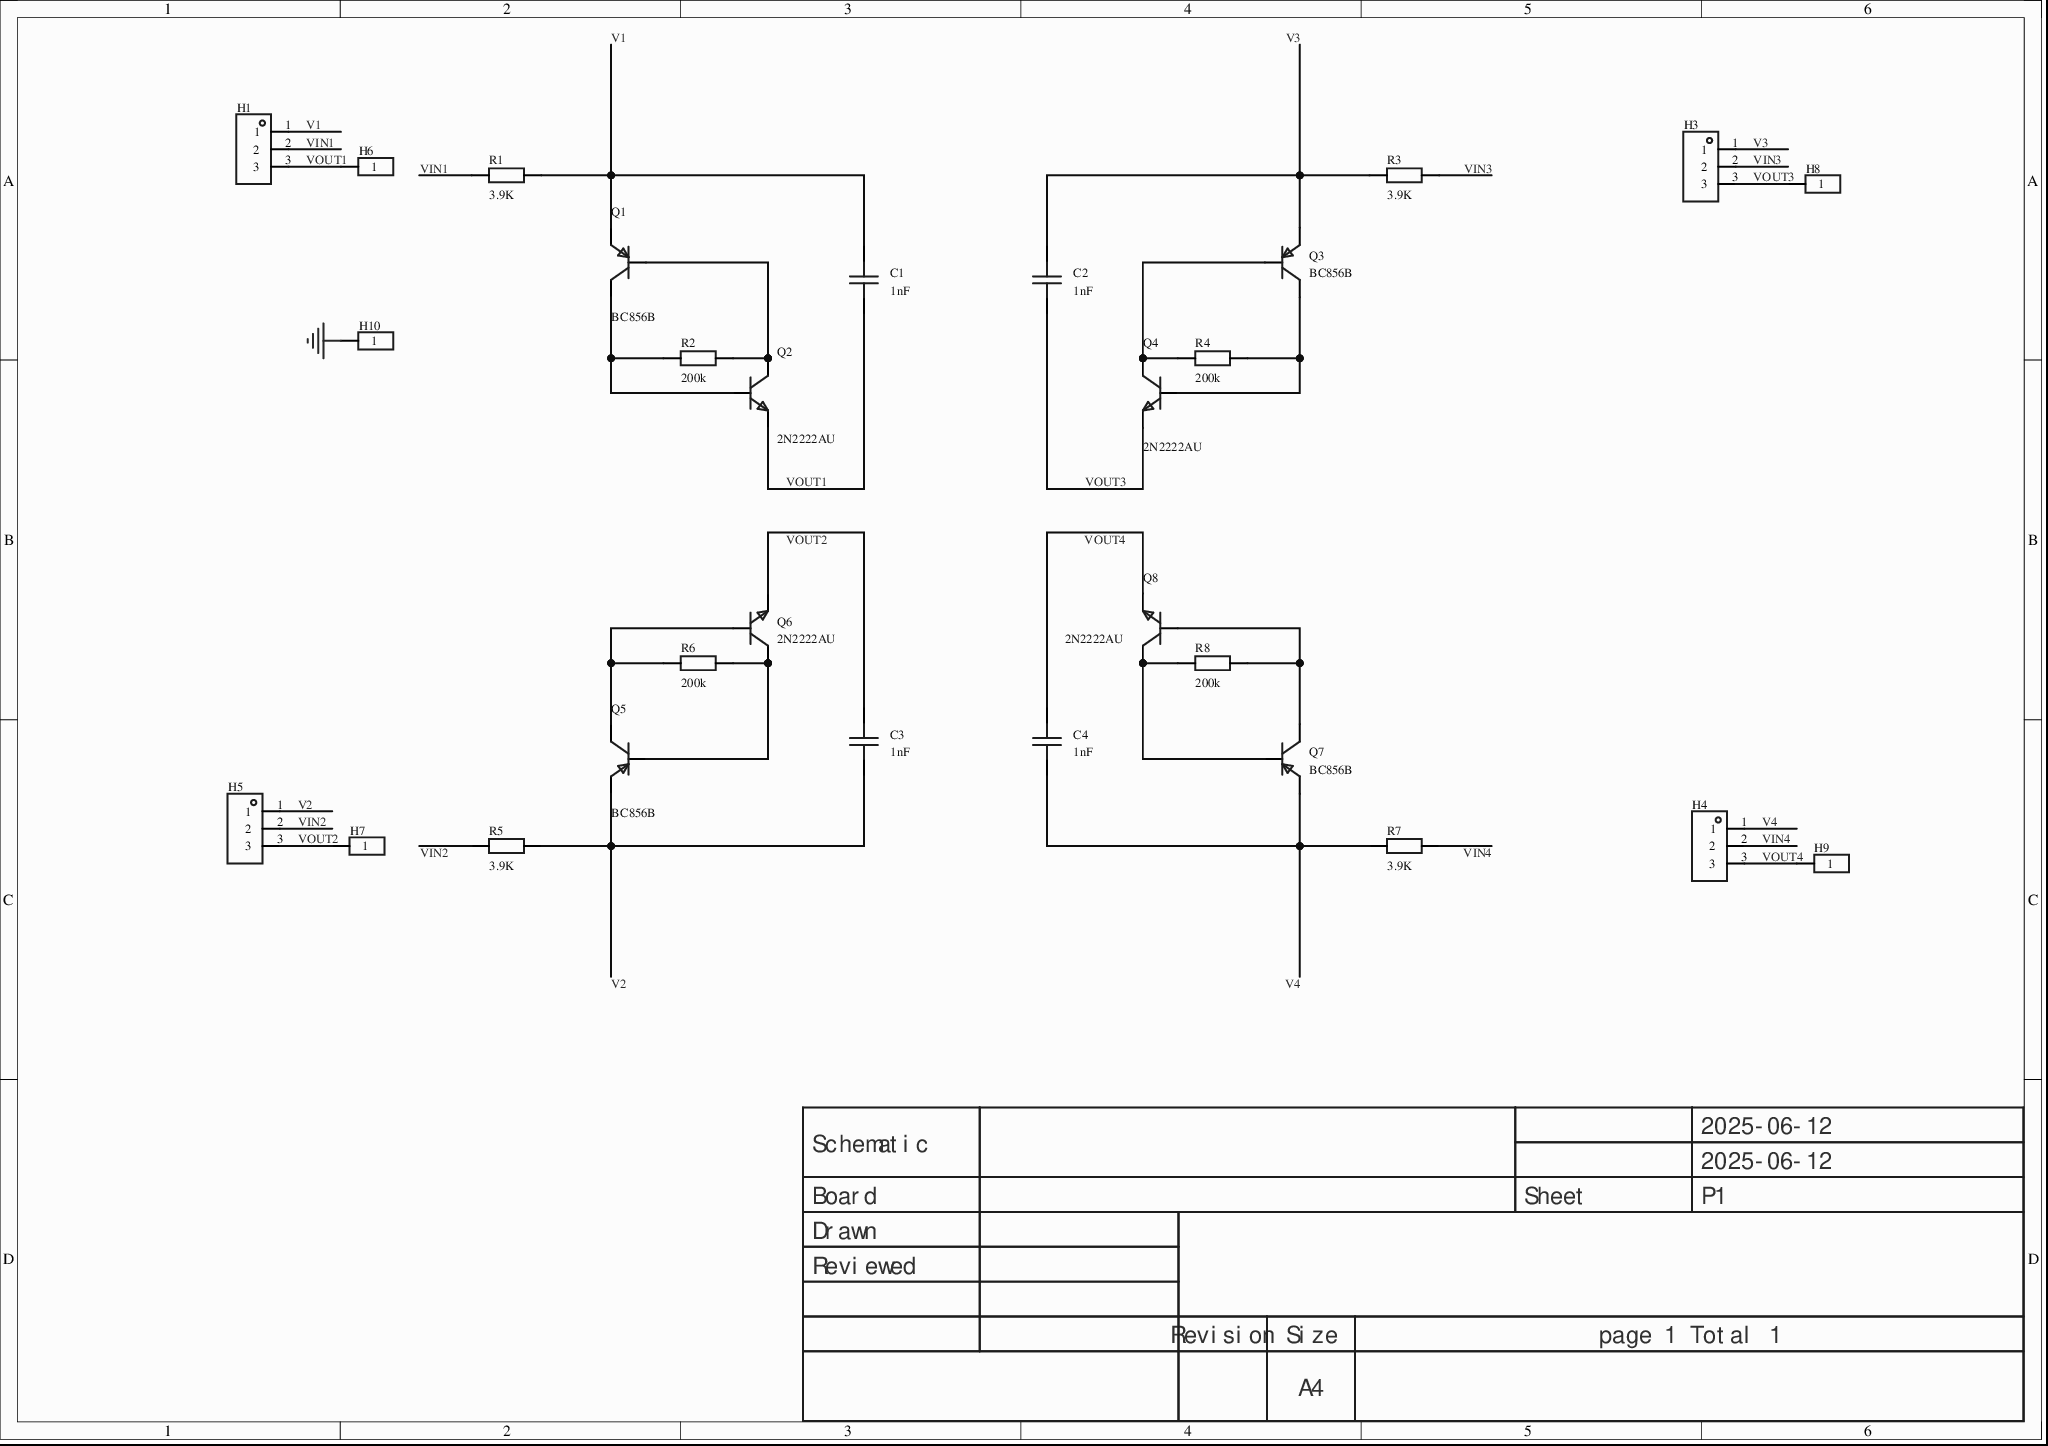
[diagram p0: MISC51650-3.schdoc]
# Altium project MISC51650-2.PrjPcb
1 sheet, 29 parts. Net scope: global (net labels, ports and power ports of the same name join across sheets).
Board file: MISC51650.pcbdoc

## Sheet MISC51650-3.schdoc
size 297 x 209 mm; Version: V1.0; @Project Name: MISC51650; @Page Count: 1; @Update Date: 2025-06-12; @Create Date: 2025-06-12; @Schematic Name: MISC51650; @Page No: 1; @Create Time: 12:37:26; @Update Time: 12:37:29; @Board Name: MISC51650

### Parts
C1  1nF  [C0402]
C2  1nF  [C0402]
C3  1nF  [C0402]
C4  1nF  [C0402]
H1  (no value)  [HDR-TH_2P-P2.54-V-M-1]
H3  (no value)  [HDR-TH_2P-P2.54-V-M-1]
H4  (no value)  [HDR-TH_2P-P2.54-V-M-1]
H5  (no value)  [HDR-TH_2P-P2.54-V-M-1]
H6  (no value)  [HDR-TH_1P-V-M_XKB_X4611WV-01I-C28D40]
H7  (no value)  [HDR-TH_1P-V-M_XKB_X4611WV-01I-C28D40]
H8  (no value)  [HDR-TH_1P-V-M_XKB_X4611WV-01I-C28D40]
H9  (no value)  [HDR-TH_1P-V-M_XKB_X4611WV-01I-C28D40]
H10  (no value)  [HDR-TH_1P-V-M_XKB_X4611WV-01I-C28D40]
Q1  BC856B  [SOT-23-3_L2.9-W1.6-P1.90-LS2.8-BR]
Q2  2N2222AU  [SOT-89-3_L4.5-W2.4-P1.50-LS4.0-BR]
Q3  BC856B  [SOT-23-3_L2.9-W1.6-P1.90-LS2.8-BR]
Q4  2N2222AU  [SOT-89-3_L4.5-W2.4-P1.50-LS4.0-BR]
Q5  BC856B  [SOT-23-3_L2.9-W1.6-P1.90-LS2.8-BR]
Q6  2N2222AU  [SOT-89-3_L4.5-W2.4-P1.50-LS4.0-BR]
Q7  BC856B  [SOT-23-3_L2.9-W1.6-P1.90-LS2.8-BR]
Q8  2N2222AU  [SOT-89-3_L4.5-W2.4-P1.50-LS4.0-BR]
R1  3.9K  [R0402]
R2  200k  [R0402]
R3  3.9K  [R0402]
R4  200k  [R0402]
R5  3.9K  [R0402]
R6  200k  [R0402]
R7  3.9K  [R0402]
R8  200k  [R0402]

### Nets
GND: H10.1
V1: C1.2 H1.1 Q1.2(E) R1.2
V2: C3.2 H5.1 Q5.2(E) R5.2
V3: C2.2 H3.1 Q3.2(E) R3.2
V4: C4.2 H4.1 Q7.2(E) R7.2
VIN1: H1.2 R1.1
VIN2: H5.2 R5.1
VIN3: H3.2 R3.1
VIN4: H4.2 R7.1
VOUT1: C1.1 H1.3 H6.1 Q2.2
VOUT2: C3.1 H5.3 H7.1 Q6.2
VOUT3: C2.1 H3.3 H8.1 Q4.2
VOUT4: C4.1 H4.3 H9.1 Q8.2
NetQ1_1: Q1.1(B) Q2.3 R2.2
NetQ1_3: Q1.3(C) Q2.1 R2.1
NetQ3_1: Q3.1(B) Q4.3 R4.2
NetQ3_3: Q3.3(C) Q4.1 R4.1
NetQ5_1: Q5.1(B) Q6.3 R6.2
NetQ5_3: Q5.3(C) Q6.1 R6.1
NetQ7_1: Q7.1(B) Q8.3 R8.2
NetQ7_3: Q7.3(C) Q8.1 R8.1

### Notes on the sheet
- 2025-06-12
- Schematic
- Board
- Sheet
- P1
- Drawn
- Reviewed
- Revision
- Size
- A4
- page 1 Total 1

### Library data of the parts
C1-C4 = CAP_0402: ConvertToPcb: yes; SymbolName: CapAcitance; ModelId: 36a51122f27c49738f86b3bfa98863e0; ModelName: C0402_L1.0-W0.5-H0.5; ModelTransform: 39.37,19.685,0,0,0,0,0,0,0; Value: 1nF; Device: CAP_0402; AddInBom: yes; Supplier Footprint: 0402; FootprintName: C0402
H1 H3-H5 = HDR-M_2.54_1x3P: Symbol: PZ254V-11-03P_C2937625; ConvertToPcb: yes; ModelId: bb473b6d38ff42a99216a4fcdbdcc4cb; ModelName: HDR-TH_3P-P2.54-M-LI-1X3P; ModelTransform: 299.9994,100,0,0,0,0,0,0,-118.11; Device: HDR-M_2.54_1x3P; AddInBom: yes; SupplierPart: C2937625; Supplier Footprint: 插件; FootprintName: HDR-TH_2P-P2.54-V-M-1
H6-H10 = HDR-M_2.54_1x1P: Symbol: HDR_1x1; ConvertToPcb: yes; ModelId: 95857080d3cc4057a19a22ccce05e171; ModelTransform: 78.74,79.1337,0,0,0,0,0,0,-110.236; Device: HDR-M_2.54_1x1P; AddInBom: yes; SupplierPart: C81276; Supplier Footprint: 插件; FootprintName: HDR-TH_1P-V-M_XKB_X4611WV-01I-C28D40; JLCPCB Part Class: Extended Part; ModelName: HDR-TH_1P-V-M_XKB_X4611WV-01I-C28D40
Q1 Q3 Q5 Q7 = BC856B_C181144: Transistor type: PNP; collector current (Ic): 100mA; collector-emitter breakdown voltage (Vceo): 65V; power dissipation (Pd): 200mW; DC current gain (hFE): 220@2mA,5V;; Manufacturer: Hottech(合科泰); AddInBom: yes; ModelId: 89cb27a44ab2466697082bb9fd73a7d0; ModelName: SOT-23-3L_L2.9-W1.6-H1.1-LS2.8-P0.95; ModelTransform: 114.173,110.236,0,90,0,0,0,0,0; Transition frequency(fT): 100MHz; Current - Collector Cutoff: 100nA; Vce Saturation(VCE(sat)): 500mV; Symbol: BC856B_C181144; Device: BC856B_C181144; LCSC Part Name: BC856B; SupplierPart: C181144; ManufacturerPart: BC856B; Supplier Footprint: SOT-23; JLCPCB Part Class: Extended library; Datasheet: https://atta.szlcsc.com/upload/public/pdf/source/20220506/36890928A961043A8557960C54EC9FEA.pdf; Supplier: LCSC; ConvertToPcb: yes; FootprintName: SOT-23-3_L2.9-W1.6-P1.90-LS2.8-BR; type: PNP; Current - Collector(Ic): 100mA; Collector - Emitter Voltage VCEO: 65V; Pd - Power Dissipation: 200mW; DC Current Gain: 220@2mA,5V; Operating Temperature: -
Q2 Q4 Q6 Q8 = 2N2222AU: Manufacturer: CBI(创基); AddInBom: yes; ModelId: dde435042bae4b9691e74da94cf9d9f3; ModelTransform: 177.165,161.417,0,90,0,0,-2.323,0,0; Symbol: 2N2222AU; Device: 2N2222AU; LCSC Part Name: 2N2222AU; SupplierPart: C21714170; ManufacturerPart: 2N2222AU; Supplier Footprint: SOT-89; JLCPCB Part Class: Extended library; Datasheet: https://atta.szlcsc.com/upload/public/pdf/source/20240307/3DBBF7265193D2D4CDAA5BD73FF82DD6.pdf; Supplier: LCSC; ConvertToPcb: yes; FootprintName: SOT-89-3_L4.5-W2.4-P1.50-LS4.0-BR; ModelName: SOT-89-3_L4.5-W2.4-P1.50-LS4.0-BR
R1-R8 = Res_0402: Symbol: Resistor; ConvertToPcb: yes; ModelId: 671aefced39d4c318694bba8bd8efd39; ModelName: R0402_L1.0-W0.5-H0.5; ModelTransform: 39.37,19.685,0,0,0,0,0,0.0005,0; Device: Res_0402; AddInBom: yes; Supplier Footprint: 0402; FootprintName: R0402
  R1 R3 R5 R7: Value: 3.9K
  R2 R4 R6 R8: Value: 200k